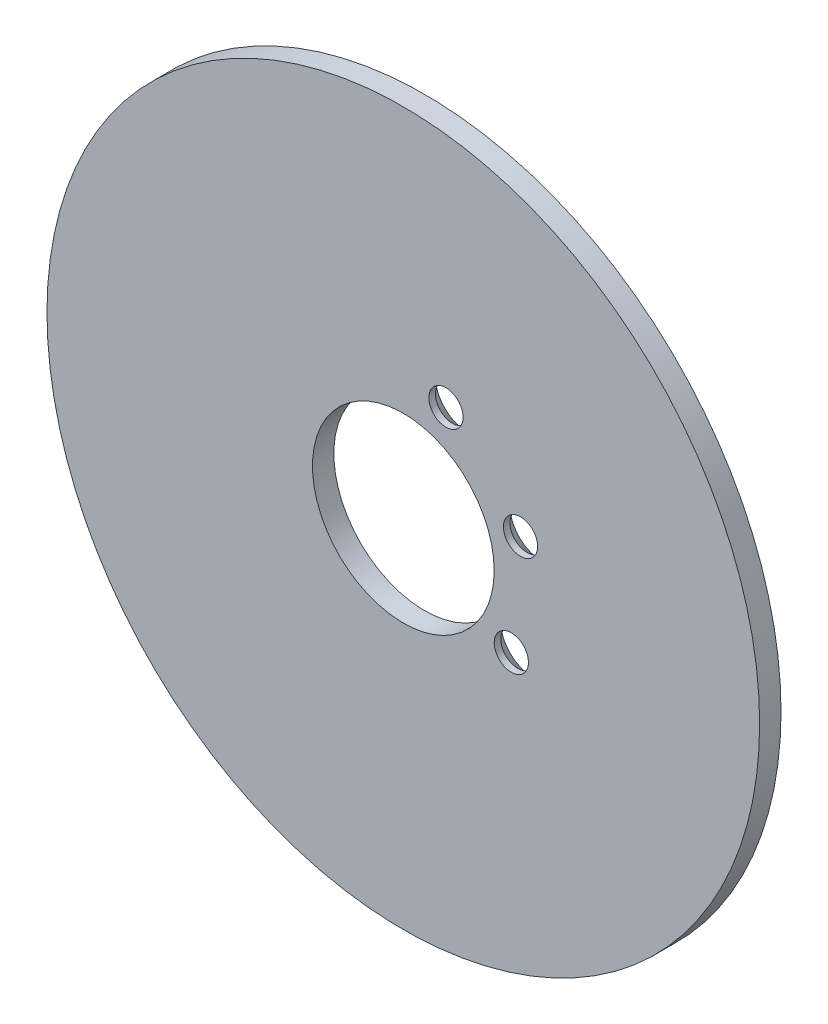
SolidWorks part; units mm, degrees
ref_plane "Front" through (0, 0, 0) normal (0, 0, 1) x (1, 0, 0)
ref_plane "Top" through (0, 0, 0) normal (0, 1, 0) x (1, 0, 0)
ref_plane "Right" through (0, 0, 0) normal (1, 0, 0) x (0, 0, -1)
sketch "Sketch1" plane through (0, 0, 0) normal (0, 0, 1) x (1, 0, 0)
  circle A0 centre (0, 0) radius 50
  circle A1 centre (0, 0) radius 12.75
  dimension "D1" = 100
  dimension "D2" = 25.5
extrude "Boss-Extrude1" add sketch "Sketch1" along normal blind 3
hole_wizard "CSK for M4 Hex Socket Countersunk Cap Screw1" positions "Sketch3" profile "Sketch2" countersink size "M4" standard "Iso" end condition through all
sketch "Sketch3" plane through (-34.7369, 24.86, 0) normal (0, 0, 1) x (1, 0, 0)
  line L0 (34.7369, -24.86) -> (40.7222, -8.4154) construction
  line L2 (34.7369, -24.86) -> (49.8923, -33.61) construction
  line L4 (34.7369, -24.86) -> (64.2189, -24.86) construction
  line L5 (34.7369, -24.86) -> (51.1815, -18.8746) construction
  circle A0 centre (34.7369, -24.86) radius 17.5 construction
  point P0 (40.7222, -8.4154)
  point P2 (49.8923, -33.61)
  point P23 (51.1815, -18.8746)
  dimension "D1" = 35
  dimension "D2" = 70
  dimension "D3" = 30
  dimension "D4" = 50
sketch "Sketch2" plane through (5.9854, 16.4446, 0) normal (1, 0, 0) x (0, 1, 0)
  line L0 (0, 0) -> (0, 3)
  line L1 (0, 3) -> (2.4, 3)
  line L2 (2.4, 3) -> (2.4, 2.08)
  line L3 (2.4, 2.08) -> (4.48, 0)
  line L5 (4.48, 0) -> (0, 0)
  line L6 (-2.4, 2.08) -> (-4.48, 0) construction
  line L11 (0, -6.35) -> (0, 107.95) construction
  dimension "通孔孔直径" = 4.8
  dimension "通孔孔深度" = 3
  dimension "近端锥形沉头孔直径" = 8.96
  dimension "近端锥形沉头孔角度" = 90
